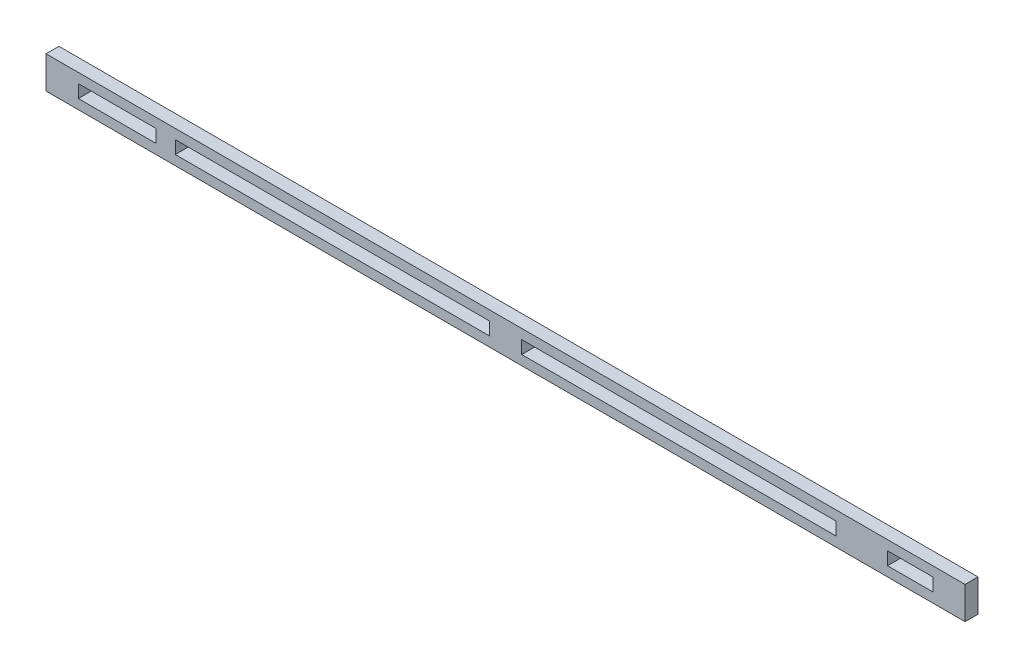
SolidWorks part; units mm, degrees
ref_plane "Front Plane" through (0, 0, 0) normal (0, 0, 1) x (1, 0, 0)
ref_plane "Top Plane" through (0, 0, 0) normal (0, 1, 0) x (1, 0, 0)
ref_plane "Right Plane" through (0, 0, 0) normal (1, 0, 0) x (0, 0, -1)
other "Configuration Table"
sketch "Sketch1" plane through (0, 0, 0) normal (0, 0, 1) x (1, 0, 0)
  line L1 (7110, -250) -> (-7110, -250)
  line L2 (7110, -250) -> (7110, 250)
  line L3 (7110, 250) -> (-7110, 250)
  line L4 (-7110, -250) -> (-7110, 250)
  line L5 (7110, -250) -> (-7110, 250) construction
  line L6 (7110, 250) -> (-7110, -250) construction
  point P0 (0, 0)
  dimension "D1" = 500
  dimension "D2" = 14220
extrude "Boss-Extrude1" add sketch "Sketch1" along normal blind 200
sketch "Sketch2" plane through (0, 0, 200) normal (0, 0, 1) x (1, 0, 0)
  line L0 (0, 0) -> (0, 1038.6166) construction
  line L1 (-6610, 100) -> (-5410, 100)
  line L2 (-6610, 100) -> (-6610, -100)
  line L3 (-6610, -100) -> (-5410, -100)
  line L4 (-5410, 100) -> (-5410, -100)
  line L5 (-5110, 100) -> (-250, 100)
  line L6 (-5110, 100) -> (-5110, -100)
  line L7 (-5110, -100) -> (-250, -100)
  line L8 (-250, 100) -> (-250, -100)
  line L9 (-7110, 0) -> (757.7523, 0) construction
  line L10 (-7110, 250) -> (-7110, -250) construction
  line L11 (250, 100) -> (250, -100)
  line L12 (5110, -100) -> (250, -100)
  line L13 (5110, 100) -> (5110, -100)
  line L14 (5110, 100) -> (250, 100)
  line L15 (5410, 100) -> (5410, -100)
  line L16 (6610, -100) -> (5410, -100)
  line L17 (6610, 100) -> (6610, -100)
  line L18 (6610, 100) -> (5410, 100)
  dimension "D1" = 200
  dimension "D2" = 500
  dimension "D3" = 300
  dimension "D4" = 1200
  dimension "D5" = 500
extrude "Cut-Extrude1" cut sketch "Sketch2" against normal through all
sketch "Sketch4" plane through (0, 0, 200) normal (0, 0, 1) x (1, 0, 0)
  line L0 (5410, -100) -> (6610, -100) construction
  line L1 (5410, 100) -> (5910, 100)
  line L2 (5410, 100) -> (5410, -100)
  line L3 (5410, -100) -> (5910, -100)
  line L4 (5910, 100) -> (5910, -100)
  dimension "D1" = 500
extrude "Boss-Extrude2" add sketch "Sketch4" against normal up to surface (200 mm away) up to face at (-6010, 0, 0)
